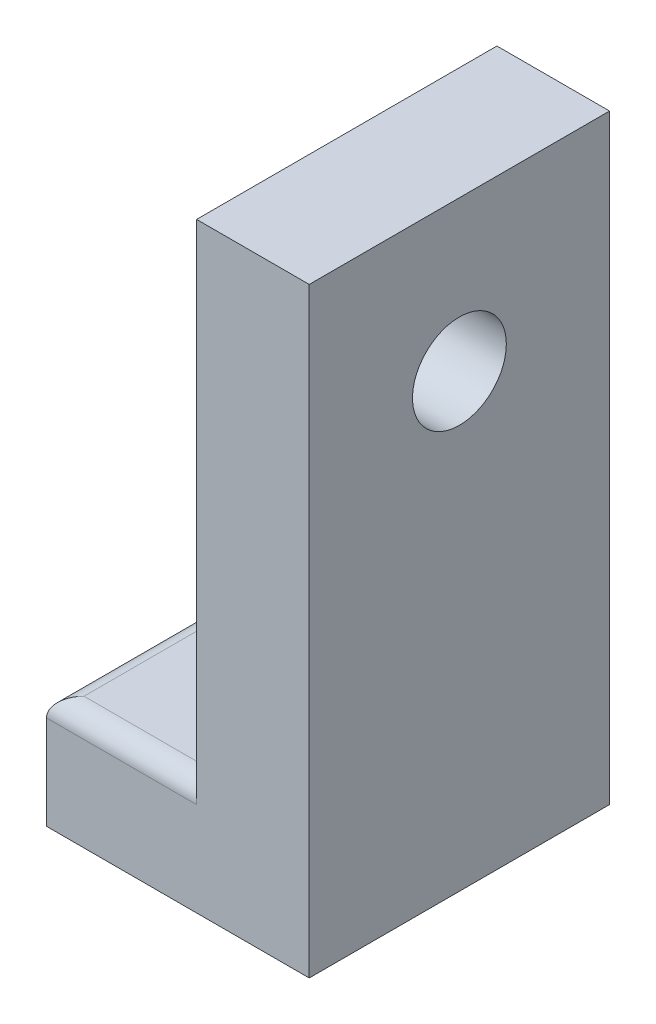
SolidWorks part; units mm, degrees
ref_plane "前视基准面" through (0, 0, 0) normal (0, 0, 1) x (1, 0, 0)
ref_plane "上视基准面" through (0, 0, 0) normal (0, 1, 0) x (1, 0, 0)
ref_plane "右视基准面" through (0, 0, 0) normal (1, 0, 0) x (0, 0, -1)
sketch "草图1" plane through (0, 0, 0) normal (0, 0, 1) x (1, 0, 0)
  line L0 (-4, -16) -> (3, -16)
  line L1 (0, 0) -> (3, 0)
  line L2 (0, 0) -> (0, -13)
  line L4 (3, 0) -> (3, -16)
  line L7 (0, -13) -> (-4, -13)
  line L8 (-4, -16) -> (-4, -13)
  dimension "D1" = 3
  dimension "D2" = 16
  dimension "D3" = 3
  dimension "D4" = 7
extrude "凸台-拉伸1" add sketch "草图1" along normal blind 8
hole_wizard "M3 螺纹孔1" positions "草图3" profile "草图2" tap size "M3" standard "Iso" end condition through all
sketch "草图3" plane through (3, 0, 0) normal (1, 0, 0) x (0, 0, -1)
  line L0 (-8, 0) -> (0, 0) construction
  point P0 (-4, -4)
  dimension "D1" = 4
sketch "草图2" plane through (3, -4, 4) normal (0, 1, 0) x (0, 0, -1)
  line L0 (0, 0) -> (0, 7)
  line L1 (0, 7) -> (1.25, 7)
  line L2 (1.25, 7) -> (1.25, 0)
  line L5 (1.25, 0) -> (0, 0)
  line L11 (0, -6.35) -> (0, 107.95) construction
  dimension "通孔螺纹孔钻头直径" = 2.5
  dimension "通孔螺纹孔钻头深度" = 7
cosmetic thread "孔螺蚊线1"
fillet "圆角1" radius 0.5 3 edges at (-2, -13, 0) (-4, -13, 4) (-2, -13, 8)
